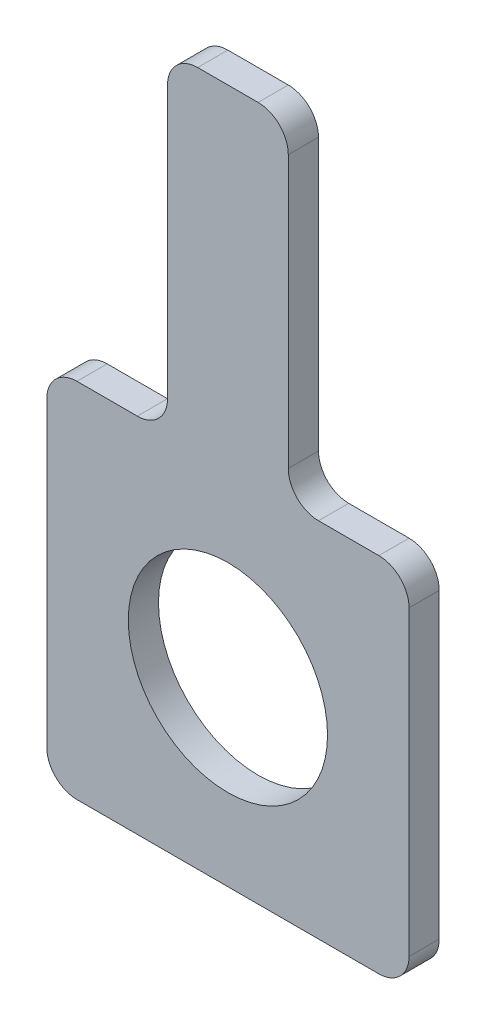
SolidWorks part; units mm, degrees
material "AISI 304"
ref_plane "Front Plane" through (0, 0, 0) normal (0, 0, 1) x (1, 0, 0)
ref_plane "Top Plane" through (0, 0, 0) normal (0, 1, 0) x (1, 0, 0)
ref_plane "Right Plane" through (0, 0, 0) normal (1, 0, 0) x (0, 0, -1)
sketch "Sketch1" plane through (0, 0, 0) normal (0, 0, 1) x (1, 0, 0)
  line L0 (2, 6) -> (6, 6)
  line L1 (-6, 6) -> (-2, 6)
  line L2 (-6, 6) -> (-6, -6)
  line L3 (-6, -6) -> (6, -6)
  line L4 (6, 6) -> (6, -6)
  line L5 (-6, 6) -> (6, -6) construction
  line L6 (-6, -6) -> (6, 6) construction
  line L8 (-2, 6) -> (-2, 17)
  line L9 (-2, 17) -> (2, 17)
  line L10 (2, 6) -> (2, 17)
  line L11 (0, 17) -> (0, 0) construction
  point P0 (0, 0)
  dimension "D1" = 12
  dimension "D2" = 12
  dimension "D3" = 4
  dimension "D4" = 11
extrude "Boss-Extrude1" add sketch "Sketch1" along normal blind 1
hole_wizard "M6 Clearance Hole1" positions "Sketch2" profile "Sketch3" hole size "M6" standard "GB" end condition through all
sketch "Sketch2" plane through (0, 0, 1) normal (0, 0, 1) x (1, 0, 0)
  point P0 (0, 0)
sketch "Sketch3" plane through (0, 0, 1) normal (1, 0, 0) x (0, -1, 0)
  line L0 (0, 0) -> (0, 1)
  line L1 (0, 1) -> (3.3, 1)
  line L2 (3.3, 1) -> (3.3, 0)
  line L5 (3.3, 0) -> (0, 0)
  line L11 (0, -6.35) -> (0, 107.95) construction
  dimension "通孔孔直径" = 6.6
  dimension "通孔孔深度" = 1
fillet "Fillet1" radius 1 8 edges at (-6, 6, 0.5) (-6, -6, 0.5) (6, -6, 0.5) (6, 6, 0.5) (2, 6, 0.5) (-2, 6, 0.5) (-2, 17, 0.5) (2, 17, 0.5)
